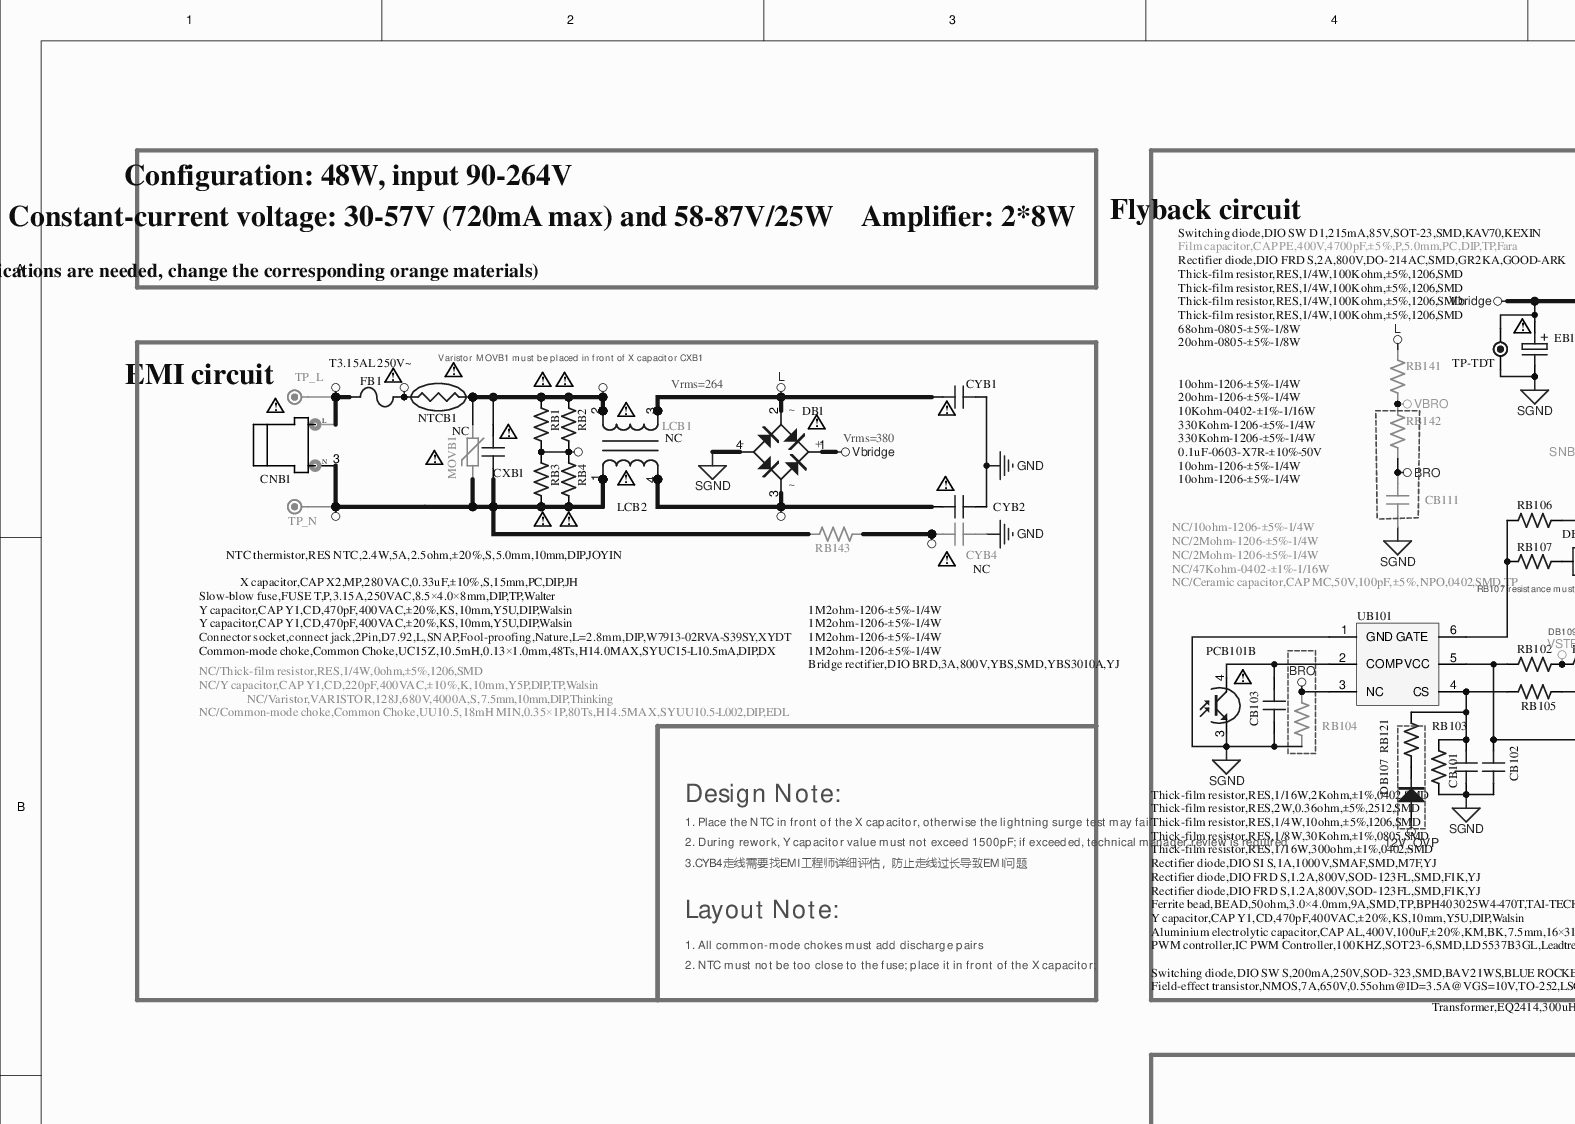
[diagram p0: MISC86372-5.SchDoc, top left]
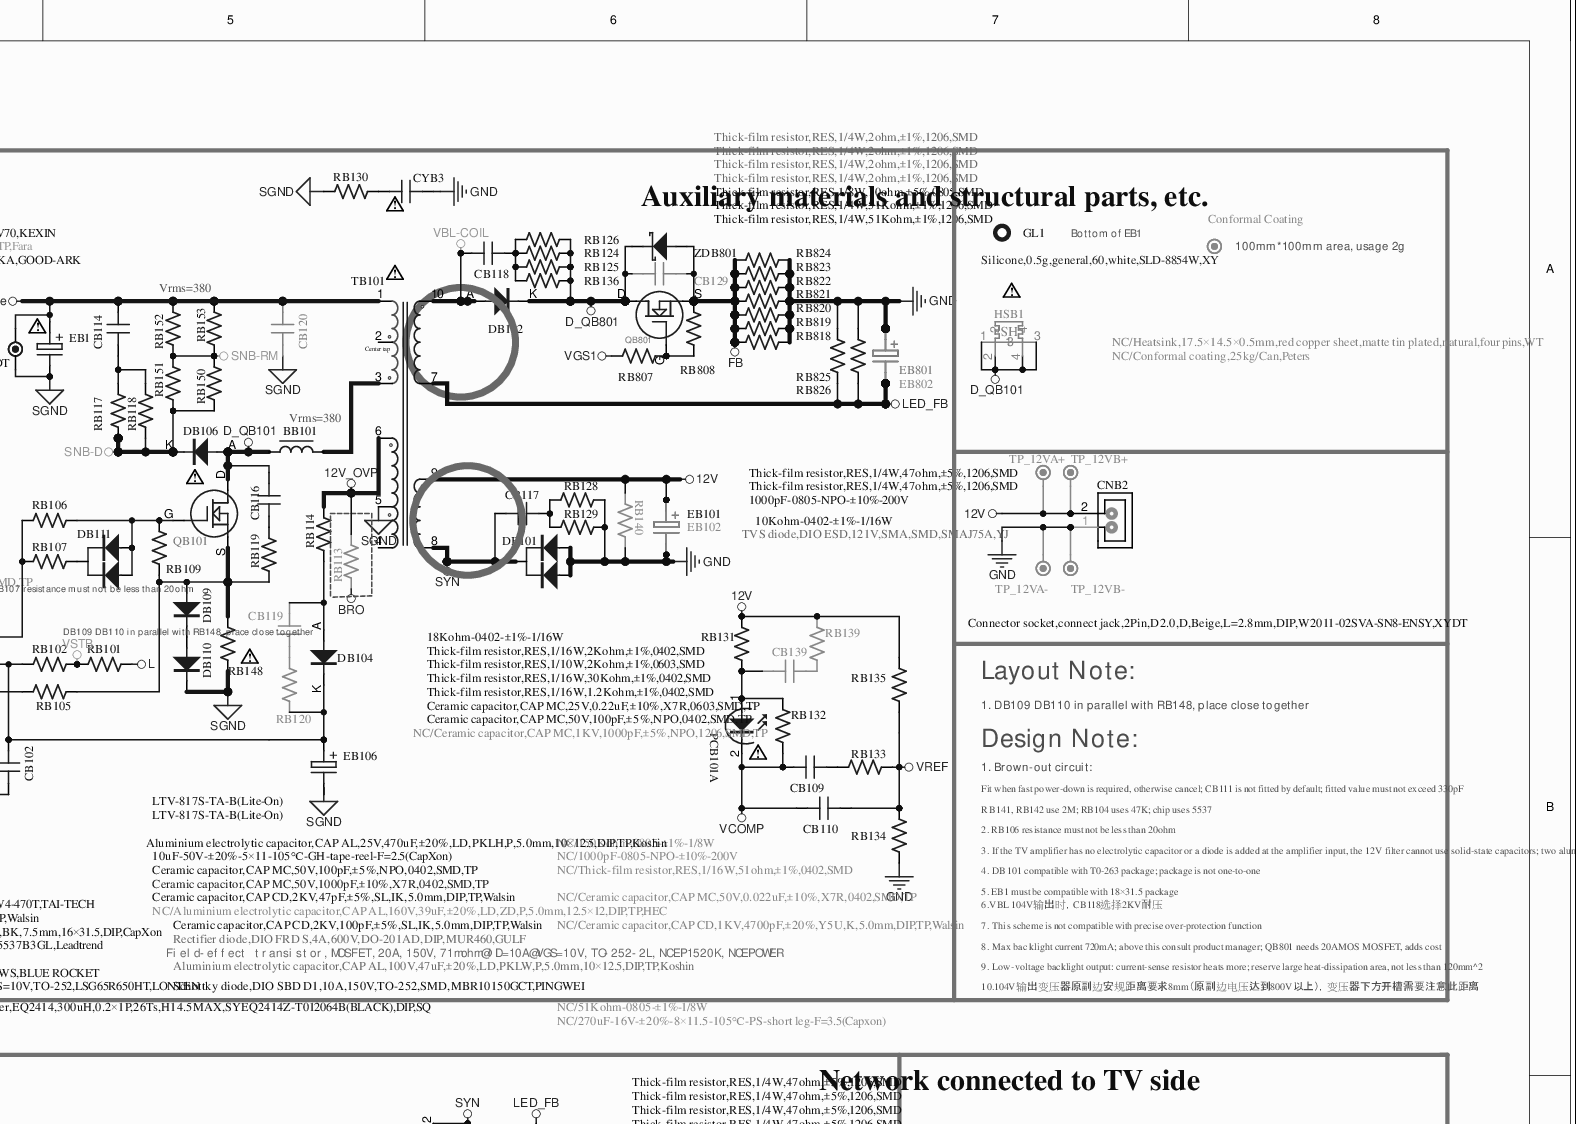
[diagram p1: MISC86372-5.SchDoc, top right]
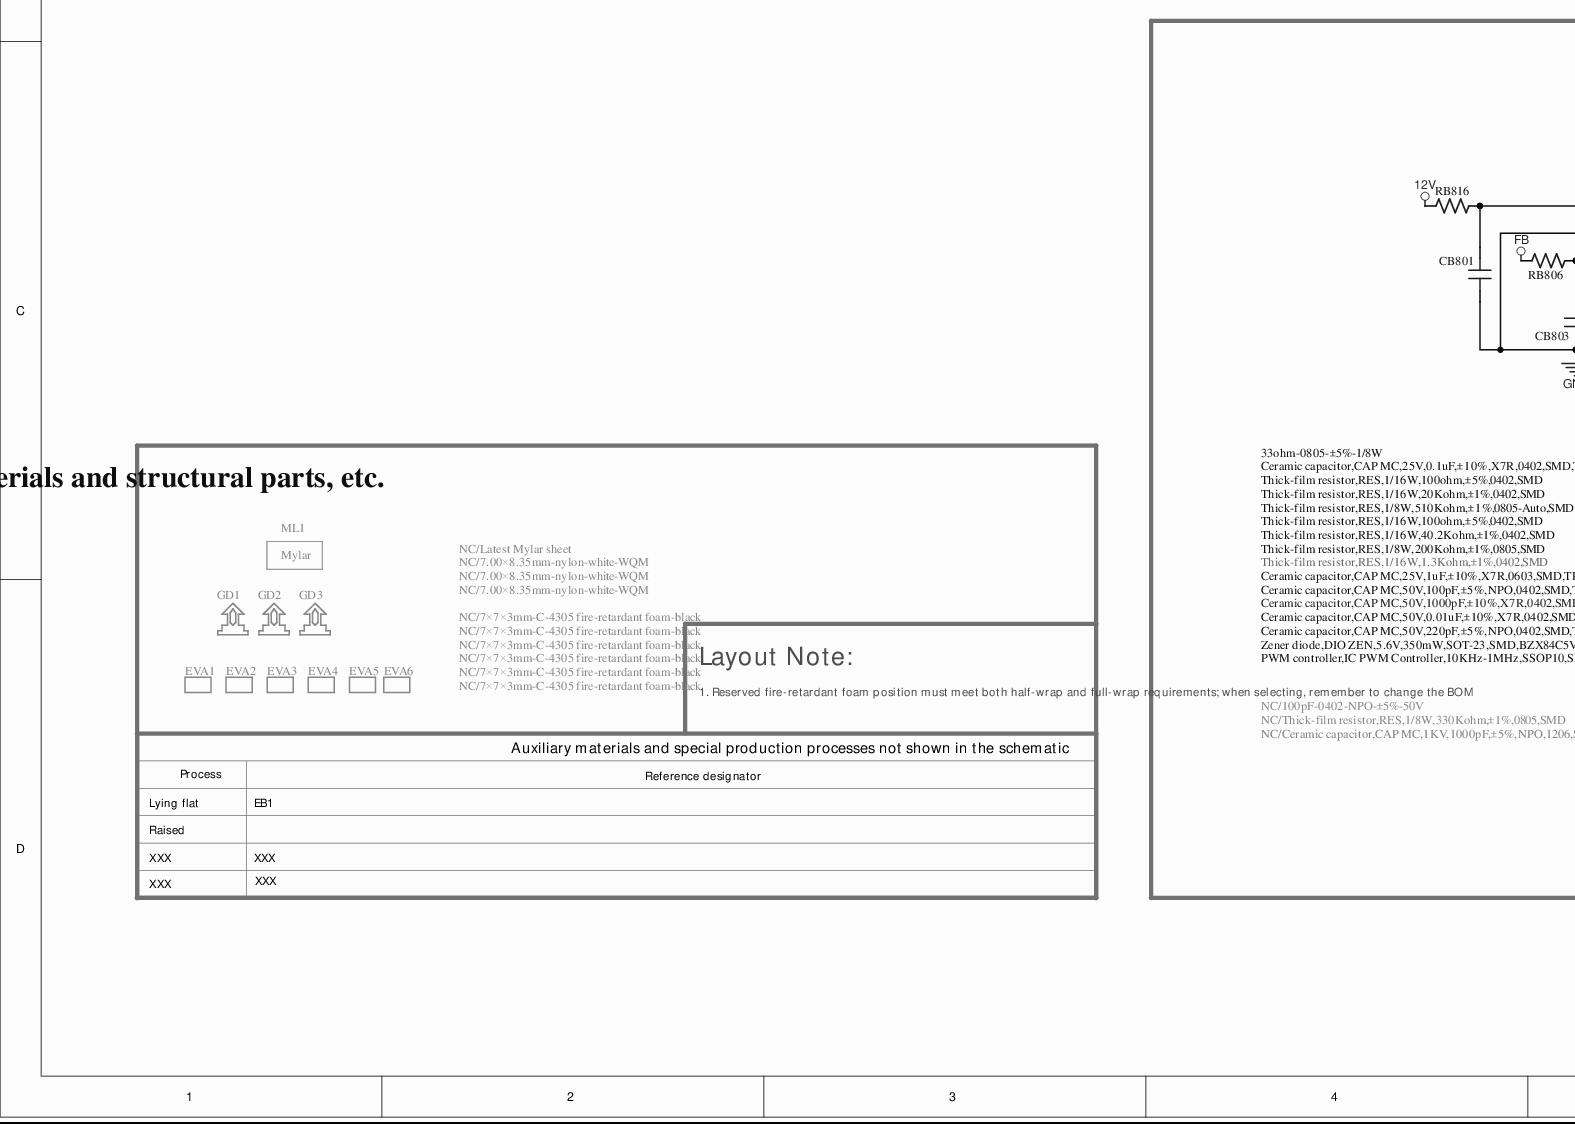
[diagram p2: MISC86372-5.SchDoc, bottom left]
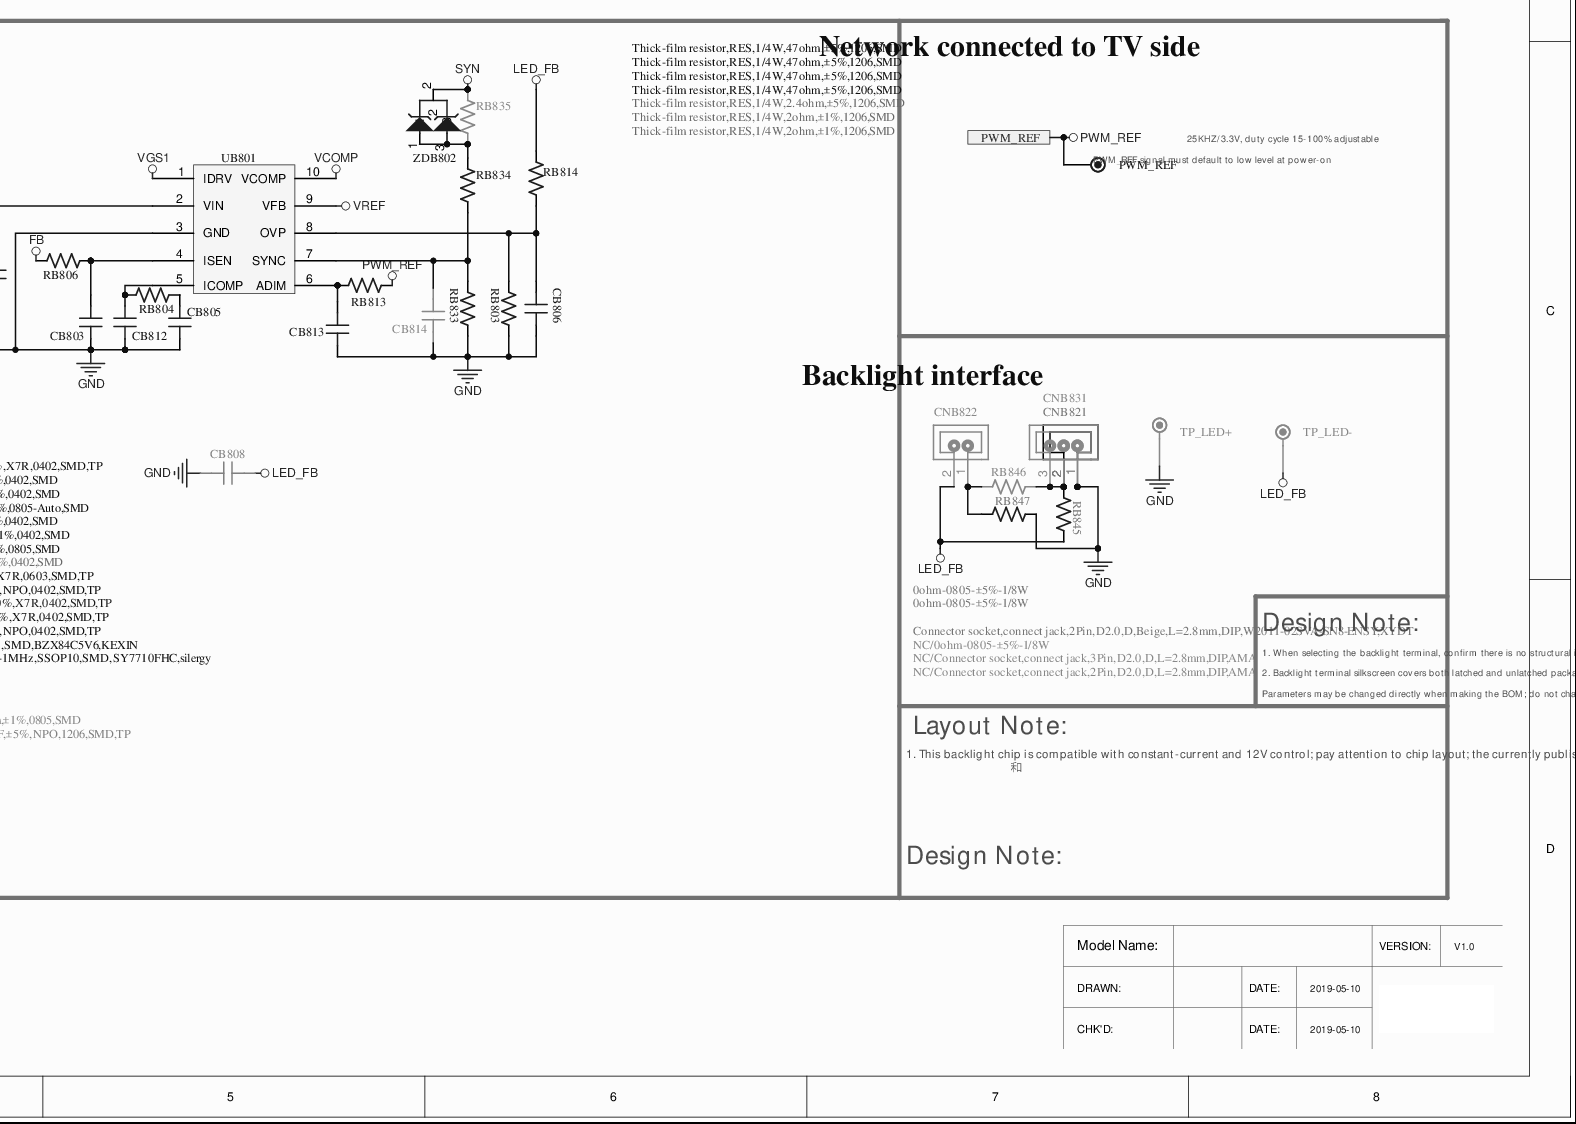
[diagram p3: MISC86372-5.SchDoc, bottom right]
# Altium project MISC86372-32.PrjPCB (part 7 of 8)

## Sheet MISC86372-5.SchDoc: MISC86372
size A2

### Parts
BB101  Ferrite bead,BEAD,50ohm,3.0×4.0mm,9A,SMD,TP,BPH403025W4-470T,TAI-TECH  [L(4*3*2.55)-S]
CB101  Ceramic capacitor,CAP MC,50V,100pF,±5%,NPO,0402,SMD,TP  [C0402]
CB102  0.1uF-0603-X7R-±10%-50V  [C0603]
CB103  Ceramic capacitor,CAP MC,50V,1000pF,±10%,X7R,0402,SMD,TP  [C0402]
CB109  Ceramic capacitor,CAP MC,25V,0.22uF,±10%,X7R,0603,SMD,TP  [C0603]
CB110  Ceramic capacitor,CAP MC,50V,100pF,±5%,NPO,0402,SMD,TP  [C0402]
CB111  NC/Ceramic capacitor,CAP MC,50V,100pF,±5%,NPO,0402,SMD,TP  [C0402]
CB114  Film capacitor,CAP PE,400V,4700pF,±5%,P,5.0mm,PC,DIP,TP,Fara  [CAP8*2.5-V-5]
CB116  Ceramic capacitor,CAP CD,2KV,47pF,±5%,SL,IK,5.0mm,DIP,TP,Walsin  [CAP7.5*5-V-5-1]
CB117  1000pF-0805-NPO-±10%-200V  [C0805]
CB118  Ceramic capacitor,CAP CD,2KV,100pF,±5%,SL,IK,5.0mm,DIP,TP,Walsin  [CAP8.5*5-V-5]
CB119  NC/1000pF-0805-NPO-±10%-200V  [C0805]
CB120  NC/Ceramic capacitor,CAP CD,1KV,4700pF,±20%,Y5U,K,5.0mm,DIP,TP,Walsin  [CAP10*4.5-V-5]
CB129  NC/Ceramic capacitor,CAP MC,1KV,1000pF,±5%,NPO,1206,SMD,TP  [C1206]
CB139  NC/Ceramic capacitor,CAP MC,50V,0.022uF,±10%,X7R,0402,SMD,TP  [C0603]
CB801  Ceramic capacitor,CAP MC,25V,1uF,±10%,X7R,0603,SMD,TP  [C0603]
CB803  Ceramic capacitor,CAP MC,25V,0.1uF,±10%,X7R,0402,SMD,TP  [C0402]
CB805  Ceramic capacitor,CAP MC,50V,0.01uF,±10%,X7R,0402,SMD,TP  [C0402]
CB806  Ceramic capacitor,CAP MC,50V,1000pF,±10%,X7R,0402,SMD,TP  [C0402]
CB808  NC/Ceramic capacitor,CAP MC,1KV,1000pF,±5%,NPO,1206,SMD,TP  [C1206]
CB812  Ceramic capacitor,CAP MC,50V,220pF,±5%,NPO,0402,SMD,TP  [C0402]
CB813  Ceramic capacitor,CAP MC,50V,100pF,±5%,NPO,0402,SMD,TP  [C0402]
CB814  NC/100pF-0402-NPO-±5%-50V  [C0402]
CNB1  Connector socket,connect jack,2Pin,D7.92,L,SNAP,Fool-proofing,Nature,L=2.8mm,DIP,W7913-02RVA-S39SY,XYDT  [CON2-H7.92]
CNB2  Connector socket,connect jack,2Pin,D2.0,D,Beige,L=2.8mm,DIP,W2011-02SVA-SN8-ENSY,XYDT  [SIP2/2.0D-1]
CNB821  Connector socket,connect jack,2Pin,D2.0,D,Beige,L=2.8mm,DIP,W2011-02SVA-SN8-ENSY,XYDT  [SIP2/2.0D-CP]
CNB822  NC/Connector socket,connect jack,2Pin,D2.0,D,L=2.8mm,DIP,AMA  [SIP2/2.0D-CP]
CNB831  NC/Connector socket,connect jack,3Pin,D2.0,D,L=2.8mm,DIP,AMA  [SIP3/2.0D-CP]
Conformal_Coating  NC/Conformal coating,25kg/Can,Peters  [Conformal Coating]
CXB1  X capacitor,CAP X2,MP,280VAC,0.33uF,±10%,S,15mm,PC,DIP,JH  [CAP18*8.5-V-15]
CYB1  Y capacitor,CAP Y1,CD,470pF,400VAC,±20%,KS,10mm,Y5U,DIP,Walsin  [CAP13*5-V-10-1]
CYB2  Y capacitor,CAP Y1,CD,470pF,400VAC,±20%,KS,10mm,Y5U,DIP,Walsin  [CAP13*5-V-10-1]
CYB3  Y capacitor,CAP Y1,CD,470pF,400VAC,±20%,KS,10mm,Y5U,DIP,Walsin  [CAP13*5-V-10-1]
CYB4  NC/Y capacitor,CAP Y1,CD,220pF,400VAC,±10%,K,10mm,Y5P,DIP,TP,Walsin  [CAP13*5-V-10-1]
DB1  Bridge rectifier,DIO BRD,3A,800V,YBS,SMD,YBS3010A,YJ  [B/YBS3010A]
DB101  Schottky diode,DIO SBD D1,10A,150V,TO-252,SMD,MBR10150GCT,PINGWEI  [D2PAK3]
DB102  Rectifier diode,DIO FRD S,4A,600V,DO-201AD,DIP,MUR460,GULF  [D3-H-20]
DB104  Rectifier diode,DIO SI S,1A,1000V,SMAF,SMD,M7F,YJ  [DIODE-S-2]
DB106  Rectifier diode,DIO FRD S,2A,800V,DO-214AC,SMD,GR2KA,GOOD-ARK  [DIODE-SMA-2]
DB107  Switching diode,DIO SW S,200mA,250V,SOD-323,SMD,BAV21WS,BLUE ROCKET  [DIODE-S-12]
DB109  Rectifier diode,DIO FRD S,1.2A,800V,SOD-123FL,SMD,F1K,YJ  [DIODE-S-14]
DB110  Rectifier diode,DIO FRD S,1.2A,800V,SOD-123FL,SMD,F1K,YJ  [DIODE-S-14]
DB111  Switching diode,DIO SW D1,215mA,85V,SOT-23,SMD,KAV70,KEXIN  [SO-23]
EB1  Aluminium electrolytic capacitor,CAP AL,400V,100uF,±20%,KM,BK,7.5mm,16×31.5,DIP,CapXon  [EC(18*31.5)-H-7.5]
EB101  Aluminium electrolytic capacitor,CAP AL,25V,470uF,±20%,LD,PKLH,P,5.0mm,10×12.5,DIP,TP,Koshin  [EC(10*12.5)-V-5]
EB102  NC/270uF-16V-±20%-8×11.5-105℃-PS-short leg-F=3.5(Capxon)  [EC(8*11)-V-3.5]
EB106  10uF-50V-±20%-5×11-105℃-GH-tape-reel-F=2.5(CapXon)  [EC(5*11)-V-2.5]
EB801  Aluminium electrolytic capacitor,CAP AL,100V,47uF,±20%,LD,PKLW,P,5.0mm,10×12.5,DIP,TP,Koshin  [EC(10*12.5)-V-5]
EB802  NC/Aluminium electrolytic capacitor,CAP AL,160V,39uF,±20%,LD,ZD,P,5.0mm,12.5×12,DIP,TP,HEC  [EC(13*13)-V-5]
EVA1  NC/7×7×3mm-C-4305 fire-retardant foam-black  [EVA(7*7*3)]
EVA2  NC/7×7×3mm-C-4305 fire-retardant foam-black  [EVA(7*7*3)]
EVA3  NC/7×7×3mm-C-4305 fire-retardant foam-black  [EVA(7*7*3)]
EVA4  NC/7×7×3mm-C-4305 fire-retardant foam-black  [EVA(7*7*3)]
EVA5  NC/7×7×3mm-C-4305 fire-retardant foam-black  [EVA(7*7*3)]
EVA6  NC/7×7×3mm-C-4305 fire-retardant foam-black  [EVA(7*7*3)]
FB1  Slow-blow fuse,FUSE T,P,3.15A,250VAC,8.5×4.0×8mm,DIP,TP,Walter  [FUSE8.5*4-V-5(T3.15AL 250V~)]
GD1  NC/7.00×8.35mm-nylon-white-WQM  [Fixed]
GD2  NC/7.00×8.35mm-nylon-white-WQM  [Fixed]
GD3  NC/7.00×8.35mm-nylon-white-WQM  [Fixed]
GL1  Silicone,0.5g,general,60,white,SLD-8854W,XY  [Silica gel-15]
HSB1  NC/Heatsink,17.5×14.5×0.5mm,red copper sheet,matte tin plated,natural,four pins,WT  [HS149-YZ]
LCB1  NC/Common-mode choke,Common Choke,UU10.5,18mH MIN,0.35×1P,80Ts,H14.5MAX,SYUU10.5-L002,DIP,EDL  [L/UU10.5/10*13-2]
LCB2  Common-mode choke,Common Choke,UC15Z,10.5mH,0.13×1.0mm,48Ts,H14.0MAX,SYUC15-L10.5mA,DIP,DX  [L/LC4/20.5*16-H-17*9(12.9)]
ML1  NC/Latest Mylar sheet  [Mylar]
MOVB1  NC/Varistor,VARISTOR,128J,680V,4000A,S,7.5mm,10mm,DIP,Thinking  [VR(13*5)-V-7.5]
NTCB1  NTC thermistor,RES NTC,2.4W,5A,2.5ohm,±20%,S,5.0mm,10mm,DIP,JOYIN  [NTC(10*5)-V5]
PCB101  LTV-817S-TA-B(Lite-On)  [OC4-S-1]  (parts A,B of 2)
PWM_REF  (no value)  [TP_BL]
QB101  Field-effect transistor,NMOS,7A,650V,0.55ohm@ID=3.5A@VGS=10V,TO-252,LSG65R650HT,LONTEN  [TO-252-GDS]
QB801  Field-effect transistor,MOSFET,20A,150V,71mohm@ID=10A@VGS=10V,TO-252-2L,NCEP1520K,NCEPOWER  [TO-252-GDS]
RB1  1M2ohm-1206-±5%-1/4W  [R1206]
RB2  1M2ohm-1206-±5%-1/4W  [R1206]
RB3  1M2ohm-1206-±5%-1/4W  [R1206]
RB4  1M2ohm-1206-±5%-1/4W  [R1206]
RB101  330Kohm-1206-±5%-1/4W  [R1206]
RB102  330Kohm-1206-±5%-1/4W  [R1206]
RB103  Thick-film resistor,RES,1/16W,2Kohm,±1%,0402,SMD  [R0402]
RB104  NC/47Kohm-0402-±1%-1/16W  [R0402]
RB105  Thick-film resistor,RES,1/16W,300ohm,±1%,0402,SMD  [R0402]
RB106  68ohm-0805-±5%-1/8W  [R0805]
RB107  20ohm-0805-±5%-1/8W  [R0805]
RB109  10Kohm-0402-±1%-1/16W  [R0402]
RB113  NC/150Kohm-0805-±1%-1/8W  [R0805]
RB114  Thick-film resistor,RES,1/4W,10ohm,±5%,1206,SMD  [R1206]
RB117  10ohm-1206-±5%-1/4W  [R1206]
RB118  10ohm-1206-±5%-1/4W  [R1206]
RB119  10ohm-1206-±5%-1/4W  [R1206]
RB120  NC/10ohm-1206-±5%-1/4W  [R1206]
RB121  Thick-film resistor,RES,1/8W,30Kohm,±1%,0805,SMD  [R0805]
RB124  Thick-film resistor,RES,1/4W,47ohm,±5%,1206,SMD  [R1206]
RB125  Thick-film resistor,RES,1/4W,47ohm,±5%,1206,SMD  [R1206]
RB126  Thick-film resistor,RES,1/4W,47ohm,±5%,1206,SMD  [R1206]
RB128  Thick-film resistor,RES,1/4W,47ohm,±5%,1206,SMD  [R1206]
RB129  Thick-film resistor,RES,1/4W,47ohm,±5%,1206,SMD  [R1206]
RB130  20ohm-1206-±5%-1/4W  [R1206]
RB131  Thick-film resistor,RES,1/10W,2Kohm,±1%,0603,SMD  [R0603]
RB132  Thick-film resistor,RES,1/16W,1.2Kohm,±1%,0402,SMD  [R0402]
RB133  Thick-film resistor,RES,1/16W,30Kohm,±1%,0402,SMD  [R0402]
RB134  Thick-film resistor,RES,1/16W,2Kohm,±1%,0402,SMD  [R0402]
RB135  18Kohm-0402-±1%-1/16W  [R0402]
RB136  Thick-film resistor,RES,1/4W,47ohm,±5%,1206,SMD  [R1206]
RB139  NC/Thick-film resistor,RES,1/16W,51ohm,±1%,0402,SMD  [R0402]
RB140  NC/51Kohm-0805-±1%-1/8W  [R0805]
RB141  NC/2Mohm-1206-±5%-1/4W  [R1206]
RB142  NC/2Mohm-1206-±5%-1/4W  [R1206]
RB143  NC/Thick-film resistor,RES,1/4W,0ohm,±5%,1206,SMD  [R1206]
RB148  Thick-film resistor,RES,2W,0.36ohm,±5%,2512,SMD  [R2512-1]
RB150  Thick-film resistor,RES,1/4W,100Kohm,±5%,1206,SMD  [R1206]
RB151  Thick-film resistor,RES,1/4W,100Kohm,±5%,1206,SMD  [R1206]
RB152  Thick-film resistor,RES,1/4W,100Kohm,±5%,1206,SMD  [R1206]
RB153  Thick-film resistor,RES,1/4W,100Kohm,±5%,1206,SMD  [R1206]
RB803  Thick-film resistor,RES,1/16W,1.3Kohm,±1%,0402,SMD  [R0402]
RB804  Thick-film resistor,RES,1/16W,20Kohm,±1%,0402,SMD  [R0402]
RB806  Thick-film resistor,RES,1/16W,100ohm,±5%,0402,SMD  [R0402]
RB807  Thick-film resistor,RES,1/8W,10ohm,±5%,0805,SMD  [R0805]
RB808  10Kohm-0402-±1%-1/16W  [R0402]
RB813  Thick-film resistor,RES,1/16W,100ohm,±5%,0402,SMD  [R0402]
RB814  Thick-film resistor,RES,1/8W,510Kohm,±1%,0805-Auto,SMD  [R0805]
RB816  33ohm-0805-±5%-1/8W  [R0805]
RB818  Thick-film resistor,RES,1/4W,2ohm,±1%,1206,SMD  [R1206]
RB819  Thick-film resistor,RES,1/4W,2ohm,±1%,1206,SMD  [R1206]
RB820  Thick-film resistor,RES,1/4W,2ohm,±1%,1206,SMD  [R1206]
RB821  Thick-film resistor,RES,1/4W,2ohm,±1%,1206,SMD  [R1206]
RB822  Thick-film resistor,RES,1/4W,2ohm,±1%,1206,SMD  [R1206]
RB823  Thick-film resistor,RES,1/4W,2ohm,±1%,1206,SMD  [R1206]
RB824  Thick-film resistor,RES,1/4W,2.4ohm,±5%,1206,SMD  [R1206]
RB825  Thick-film resistor,RES,1/4W,51Kohm,±1%,1206,SMD  [R1206]
RB826  Thick-film resistor,RES,1/4W,51Kohm,±1%,1206,SMD  [R1206]
RB833  Thick-film resistor,RES,1/16W,40.2Kohm,±1%,0402,SMD  [R0402]
RB834  Thick-film resistor,RES,1/8W,200Kohm,±1%,0805,SMD  [R0805]
RB835  NC/Thick-film resistor,RES,1/8W,330Kohm,±1%,0805,SMD  [R0805]
RB845  0ohm-0805-±5%-1/8W  [R0805]
RB846  NC/0ohm-0805-±5%-1/8W  [R0805]
RB847  0ohm-0805-±5%-1/8W  [R0805]
TB101  Transformer,EQ2414,300uH,0.2×1P,26Ts,H14.5MAX,SYEQ2414Z-T012064B(BLACK),DIP,SQ  [T/EQ2414*10]
TP-TDT  (no value)  [TP-TDT]
TP_12VA+  NC/  [TP]  (value not drawn)
TP_12VA-  NC/  [TP]  (value not drawn)
TP_12VB+  NC/  [TP]  (value not drawn)
TP_12VB-  NC/  [TP]  (value not drawn)
TP_L  NC/  [TP-80]  (value not drawn)
TP_LED+  NC/  [TP]  (value not drawn)
TP_LED-  NC/  [TP]  (value not drawn)
TP_N  NC/  [TP-80]  (value not drawn)
UB101  PWM controller,IC PWM Controller,100KHZ,SOT23-6,SMD,LD5537B3GL,Leadtrend  [SOT-26]
UB801  PWM controller,IC PWM Controller,10KHz-1MHz,SSOP10,SMD,SY7710FHC,silergy  [SOP10/1.0-1]
ZDB801  TVS diode,DIO ESD,121V,SMA,SMD,SMAJ75A,YJ  [DIODE-SMA-1]
ZDB802  Zener diode,DIO ZEN,5.6V,350mW,SOT-23,SMD,BZX84C5V6,KEXIN  [SO-23]

### Ports
PWM_REF

### Nets
12V: CNB2.2 EB101.1 EB102.1 RB131.2 RB135.1 RB139.1 RB140.1 RB816.1 TB101.9 TP_12VA+.1 TP_12VB+.1
12V_OVP: DB107.A RB113.2 RB114.2 TB101.6
BRO: CB111.2 RB104.2 RB113.1 RB142.1 UB101.3(NC)
D_QB101: BB101.1 CB116.1 DB106.A HSB1.1 HSB1.2 HSB1.3 HSB1.4 QB101.D
D_QB801: CB129.1 DB102.K QB801.D RB124.1 RB125.1 RB126.1 RB136.1 ZDB801.K
FB: CB129.2 QB801.S RB806.1 RB808.2 RB818.1 RB819.1 RB820.1 RB821.1 RB822.1 RB823.1 RB824.1 ZDB801.A
GND: CB801.2 CB803.2 CB805.1 CB806.2 CB808.1 CB812.1 CB813.1 CB814.2 CNB2.1 CNB821.1 CNB831.1 CYB1.2 CYB2.2 CYB3.2 CYB4.2 DB101.1 DB101.3 EB101.2 EB102.2 EB801.1 EB802.1 RB128.2 RB129.2 RB134.1 RB140.2 RB803.1 RB818.2 RB819.2 RB820.2 RB821.2 RB822.2 RB823.2 RB824.2 RB825.1 RB826.1 RB833.1 RB847.1 TP_12VA-.1 TP_12VB-.1 TP_LED+.1 UB801.3(GND)
L: CYB1.1 DB1.2 LCB1.3 LCB2.3 RB101.1 RB141.2
L-1: CNB1.1 FB1.1 TP_L.1
L-2: FB1.2 NTCB1.1
L-3: CXB1.1 LCB1.2 LCB2.2 MOVB1.1 NTCB1.2 RB1.1 RB2.1
L-N: RB1.2 RB2.2 RB3.1 RB4.1
LED_FB: CB808.2 CNB822.2 EB801.2 EB802.2 RB814.1 RB825.2 RB826.2 RB845.1 TB101.7 TP_LED-.1
N-1: CNB1.3 CXB1.2 LCB1.1 LCB2.1 MOVB1.2 RB3.2 RB4.2 RB143.1 TP_N.1
N-2: CYB2.1 DB1.3 LCB1.4 LCB2.4
N-3: CYB4.1 RB143.2
PWM_REF: PWM_REF.1 RB813.1 ; port PWM_REF
SGND: CB101.2 CB102.2 CB103.2 CB111.1 CB120.1 DB1.4 DB110.K EB1.2 EB106.2 PCB101.3 RB103.1 RB104.1 RB130.1 RB148.1 TB101.5 TP-TDT.2 UB101.1(GND)
SNB-D: DB106.K RB117.1 RB118.1 RB150.1 RB151.1
SNB-RM: RB150.2 RB151.2 RB152.1 RB153.1
SYN: CB117.1 DB101.2 RB835.1 TB101.8 ZDB802.2
VBL-COIL: CB118.1 DB102.A TB101.10
Vbridge: CB114.1 CB120.2 DB1.1 EB1.1 RB152.2 RB153.2 TB101.1 TP-TDT.1
VBRO: RB141.1 RB142.2
VCOMP: CB109.1 CB110.1 PCB101.2 RB132.1 UB801.10(VCOMP)
VGS1: RB807.1 UB801.1(IDRV)
VREF: CB110.2 RB133.1 RB134.2 RB135.2 UB801.9(VFB)
VSTB: RB101.2 RB102.2
NetBB101_2: BB101.2 TB101.3
NetCB101_1: CB101.1 RB103.2 RB105.1 RB121.2 UB101.4(CS)
NetCB102_1: CB102.1 DB104.K EB106.1 RB102.1 RB120.1 UB101.5(VCC)
NetCB103_1: CB103.1 PCB101.4 UB101.2(COMP)
NetCB109_2: CB109.2 RB133.2
NetCB114_2: CB114.2 RB117.2 RB118.2
NetCB116_2: CB116.2 RB119.2
NetCB117_2: CB117.2 RB128.1 RB129.1
NetCB118_2: CB118.2 RB124.2 RB125.2 RB126.2 RB136.2
NetCB119_1: CB119.1 RB120.2
NetCB119_2: CB119.2 DB104.A RB114.1
NetCB139_1: CB139.1 RB139.2
NetCB139_2: CB139.2 PCB101.1 RB131.1 RB132.2
NetCB801_1: CB801.1 RB816.2 UB801.2(VIN)
NetCB803_1: CB803.1 RB806.2 UB801.4(ISEN)
NetCB805_2: CB805.2 RB804.1
NetCB806_1: CB806.1 RB803.2 RB814.2 UB801.8(OVP)
NetCB812_2: CB812.2 RB804.2 UB801.5(ICOMP)
NetCB813_2: CB813.2 RB813.2 UB801.6(ADIM)
NetCB814_1: CB814.1 RB833.2 RB834.1 UB801.7(SYNC)
NetCNB821_2: CNB821.2 CNB831.2 CNB831.3 RB845.2 RB846.1
NetCNB822_1: CNB822.1 RB846.2 RB847.2
NetCYB3_1: CYB3.1 RB130.2
NetDB107_K: DB107.K RB121.1
NetDB109_A: DB109.A QB101.S RB105.2 RB109.1 RB119.1 RB148.2
NetDB109_K: DB109.K DB110.A
NetDB111_1: DB111.1 DB111.3 QB101.G RB106.2 RB109.2
NetDB111_2: DB111.2 RB107.2
NetQB801_G: QB801.G RB807.2 RB808.1
NetRB106_1: RB106.1 RB107.1 UB101.6(GATE)
NetRB834_2: RB834.2 RB835.2 ZDB802.1 ZDB802.3

Not connected (* = marked no-connect by the designer): TB101 2* 4*

### Layout directives
net class HOT: 12V, 12V_OVP, BRO, D_QB101, D_QB801, FB, GND, L, L-1, L-2, L-3, L-N, LED_FB, N-1, N-2, N-3, PWM_REF, SGND, SNB-D, SNB-RM, SYN, VBL-COIL, Vbridge, VBRO, VCOMP, VGS1, VREF, VSTB
net class POWER: 12V, 12V_OVP, BRO, D_QB101, D_QB801, FB, GND, L, L-1, L-2, L-3, L-N, LED_FB, N-1, N-2, N-3, PWM_REF, SGND, SNB-D, SNB-RM, SYN, VBL-COIL, Vbridge, VBRO, VCOMP, VGS1, VREF, VSTB

### Notes on the sheet
- Configuration: 48W, input 90-264V
- Constant-current voltage: 30-57V (720mA max) and 58-87V/25W
- Amplifier: 2*8W
- Flyback circuit
- (near CYB3) !
- Bottom of EB1
- Auxiliary materials and structural parts, etc.
- (near Conformal_Coating) 100mm*100mm area, usage 2g
- (If other specifications are needed, change the corresponding orange materials)
- (near EB1) !
- Vrms=380
- (near TB101) !
- !
- (near TP_L) EMI circuit
- Varistor MOVB1 must be placed in front of X capacitor CXB1
- (near NTCB1) !
- Vrms=264
- (near MOVB1) NC
- (near CXB1) !
- NC
- (near DB1) !
- (near DB1) Vrms=380
- (near CYB1) !
- (near BB101) Vrms=380
- (near RB4) !
- (near CYB2) !
- (near QB101) !
- (near CYB4) !
- (near CYB4) NC
- (near DB109) RB107 resistance must not be less than 20ohm
- DB109 DB110 in parallel with RB148, place close together
- (near RB148) !
- 1. DB109 DB110 in parallel with RB148, place close together
- Layout Note:
- Design Note:
- 1. Brown-out circuit:
- Fit when fast power-down is required, otherwise cancel; CB111 is not fitted by default; fitted value must not exceed 330pF
- RB141, RB142 use 2M; RB104 uses 47K; chip uses 5537
- 1. Place the NTC in front of the X capacitor, otherwise the lightning surge test may fail
- (near DB107) 2. During rework, Y capacitor value must not exceed 1500pF; if exceeded, technical manager review is required
- 3.CYB4走线需要找EMI工程师详细评估，防止走线过长导致EMI问题
- 3. If the TV amplifier has no electrolytic capacitor or a diode is added at the amplifier input, the 12V filter cannot use solid-state capacitors; two aluminium electrolytics are required
- 4. DB101 compatible with T0-263 package; package is not one-to-one
- 2. RB106 resistance must not be less than 20ohm
- 1. All common-mode chokes must add discharge pairs
- 6.VBL 104V输出时，CB118选择2KV耐压
- 5. EB1 must be compatible with 18×31.5 package
- 7. This scheme is not compatible with precise over-protection function
- 8. Max backlight current 720mA; above this consult product manager; QB801 needs 20AMOS MOSFET, adds cost
- 2. NTC must not be too close to the fuse; place it in front of the X capacitor;
- 9. Low-voltage backlight output: current-sense resistor heats more; reserve large heat-dissipation area, not less than 120mm^2
- 10.104V输出变压器原副边安规距离要求8mm（原副边电压达到800V以上），变压器下方开槽需要注意此距离
- Network connected to TV side
- 25KHZ/3.3V, duty cycle 15-100% adjustable
- (near PWM_REF) PWM_REF signal must default to low level at power-on
- Backlight interface
- (near ML1) Auxiliary materials and structural parts, etc.
- 1. When selecting the backlight terminal, confirm there is no structural interference with the PCB
- 1. Reserved fire-retardant foam position must meet both half-wrap and full-wrap requirements; when selecting, remember to change the BOM
- 2. Backlight terminal silkscreen covers both latched and unlatched packages
- Parameters may be changed directly when making the BOM; do not change the package
- Process
- Auxiliary materials and special production processes not shown in the schematic
- Reference designator
- 1. This backlight chip is compatible with constant-current and 12V control; pay attention to chip layout; the currently published layout scheme may be referred to
- XXXXXXXXXXXXXXXX和XXXXXXXXXXXXXX
- Lying flat
- Raised
- XXX
- EB1
- Model Name:
- DRAWN:
- XXXXXXXXXXXXXX XXXXXX
- PERSON_A
- DATE:
- 2019-05-10
- VERSION:
- V1.0
- CHK'D:
- PERSON_B
- Title
- Size:
- Date:
- A4
- Number:
- Time:
- Revision:
- Sheet
- of
- File:

### Library data of the parts
BB101 = 磁珠,BEAD,50ohm,3.0×4.0,9A,SMD,TP,SMB-302540-K5B-L1,SOLDIER-D
CB101 CB803 CB814 = 100pF-0402-NPO-±5%-50V-D
CB102 CB109 CB139 = 0.1uF-0603-X7R-±10%-50V-D: CAP
CB103 = 1000pF-0402-X7R-±10%-50V-D
CB110 CB806 = 1000pF-0402-X7R-±10%-50V-D: CAP
CB111 = 004.003.0000501-D: Ceramic capacitor,CAP MC,50V,100pF,±5%,NPO,0402,SMD,TP-D
CB114 = C242G472J20A201(编带/法拉)-DAI: CAP
CB116 = 004.003.0001895-DHAI: Ceramic capacitor,CAP CD,2KV,100pF,±5%,SL,OK,5.0mm,DIP,TP,TDK-DHAI
CB117 CB119 = 1000pF-0805-NPO-±10%-200V-D: CAP
CB118 = 004.003.0001892-DHAI: Ceramic capacitor,CAP CD,1KV,220pF,±5%,SL,OK,5.0mm,DIP,TP,TDK-DHAI
CB120 = 004.003.0001665: Ceramic capacitor,CAP CD,1KV,4700pF,±20%,Y5U,K,5.0mm,DIP,TP,Walsin-DHAI
CB129 CB808 = 22pF-1206-NPO±5%-1000V-D
CB801 = 1uf-0603-X7R-±10%-25V-D
CB805 = 0.1uF-0402-X7R-±10%-16V-D
CB812 = 0.033uF-0402-X7R-±10%-16V-D
CB813 = 4700pF-0402-X7R-±10%-50V-D
CNB1 = 连接插座,connect jack,2Pin,D7.92,L,SNAP,Fool-proofing,nature,L=2.8mm,DIP,AMA-DLMI: AC socket
CNB2 CNB821 CNB822 = XXX.XXX.0001753: Connector socket,connect jack,2Pin,D2.0,D,L=2.8mm,DIP,AMA-DHMI
CNB831 = XXX.XXX.0001754: Connector socket,connect jack,3Pin,D2.0,D,L=2.8mm,DIP,AMA-DHMI
Conformal_Coating = 三防漆,25kg/Can,Peters
CXB1 = X电容,CAP X2,MP,275VAC,0.47uF,±10%,S,15mm-Mini,PC,DIP,BM-DHMI: CAP
CYB1-CYB4 = Y电容,CAP Y1,CD,470pF,400VAC,±20%,KS,10mm,Y5U,DIP,Walsin-DHMI: Y1 capacitor
DB1 = 004.005.0000860-D: Bridge rectifier,DIO BRD,3A,800V,YBS,SMD,YBS3010A,YJ-D
DB101 = MBRB10150CT(GOOD-ARK)-D: Diode
DB102 = 004.005.0000308: Rectifier diode,DIO UFRD S,4A,800V,DO-201AD,DIP,MUR480ERLG,ON-DLMI
DB104 = M7(WEJ)-D: Diode
DB106 = 004.005.0000504-D: Rectifier diode,DIO FRD S,2A,800V,DO-214AC,SMD,GR2KA,GOOD-ARK-D
DB107 = BAV21WS-D: Diode
DB109 DB110 = 整流二极管,DIO FRD S,1.2A,800V,eSGA,SMD,R12K,GOOD-ARK-D
DB111 = LBAV70LT1G(LRC)-D: Diode
EB1 = 铝电解电容,CAP AL,450V,68uF,±20%,KM,BK,7.5mm,18×31.5,DIP,CapXon-DLMI: CAP
EB101 = 470uF-25V-±20%-10×12.5-105℃-GF-编带-F=5.0(CapXon)-DHAI: Electrolytic
EB102 = 270uF-16V-±20%-8×11.5-105℃-PS-短脚-F=3.5(Capxon): Solid-state
EB106 = 10uF-50V-±20%-5×11-105℃-GH-编带-F=2.5(CapXon)-DHAI: Electrolytic
EB801 = 004.003.0000876: Aluminium electrolytic capacitor,CAP AL,100V,47uF,±20%,LD,SK,P,5.0mm,10×12.5,DIP,TP,Samxon-DHAI
EB802 = 004.003.0000945: Aluminium electrolytic capacitor,CAP AL,160V,39uF,±20%,LD,DV,P,5.0mm,12.5×12,DIP,TP,Elite-DHAI
EVA1-EVA6 = 7×7×3mm-C-4305防火泡棉-黑色-DLMI: EVA
FB1 = 004.026.0000010-DHMI: Slow-blow fuse,FUSE T,P,3.15A,250VAC,8.5×4.0×8mm,DIP,TP,Walter-DHMI
GD1-GD3 = 7.00×8.35mm-尼龙-白色-WQM-DHMI: Mylar standoff
GL1 = 005.002.0000011: Silicone,0.2g,general,60,white,SLD-8854W,XY-DHMI
HSB1 = 004.040.0006600-DHMI: Heatsink,17.5×14.5×0.5mm,red copper sheet,matte tin plated,natural,four pins,WT-DHMI
LCB1 = SYUU10.5-L002-JM-DHMI: Common-mode choke
LCB2 = 共模电感,Common Choke,UC15,10.5mH,0.13×1.0mm,48Ts,H14.0MAX,SYUC15-L10.5mA,DIP,UENO-DLMI: Common-mode choke
ML1 = MALAY
MOVB1 = TVR10561KSW(为勤)-DHMI: Varistor
NTCB1 = SCK102R55AMBY502(短脚/为勤)-DHMI: Thermistor
PCB101 = LTV-817S-TA-B(光宝)-DMI: Optocoupler
PWM_REF TP-TDT TP_12VA+ TP_12VA- TP_12VB+ TP_12VB- TP_L TP_LED+ TP_LED- TP_N = TEST
QB101 = 场效应管,NMOS,5.2,650V,1.02ohm@ID=2.6A@VGS=10V,DPAK,TK5P65W,TOSHIBA-D: N Channel Single MOSFET
QB801 = ME15N10(松木)-D: N Channel Single MOSFET
RB1-RB4 = 1M2ohm-1206-±5%-1/4W-D: RES
RB101 RB102 = 330Kohm-1206-±5%-1/4W-D: RES
RB103 RB109 RB808 = 10Kohm-0402-±1%-1/16W-D
RB104 = 47Kohm-0402-±1%-1/16W-D
RB105 = 510ohm-0402-±1%-1/16W-D
RB106 RB113 RB121 = 68ohm-0805-±5%-1/8W-D
RB107 RB807 = 20ohm-0805-±5%-1/8W-D: RES
RB114 = 4R7ohm-1206-±1%-1/4W-D: RES
RB117-RB120 = 10ohm-1206-±5%-1/4W-D: RES
RB124-RB126 RB136 = 68ohm-1206-±5%-1/4W-D
RB128 RB129 = 47ohm-1206-±5%-1/4W-D: RES
RB130 RB143 = 20ohm-1206-±5%-1/4W-D
RB131 = 2Kohm-0603-±5%-1/10W-D
RB132 RB133 RB139 = 3Kohm-0402-±1%-1/16W-D
RB134 = 4K7ohm-0402-±1%-1/16W-D: RES
RB135 = 18Kohm-0402-±1%-1/16W-D: RES
RB140 = 51Kohm-0805-±1%-1/8W-D: RES
RB141 RB142 = 2Mohm-1206-±5%-1/4W-D: RES
RB148 = 厚膜电阻,RES,1W,0.24ohm,±1%,2512,SMD
RB150-RB153 RB825 RB826 = 100Kohm-1206-±5%-1/4W-D: RES
RB803 RB813 RB833 = 100ohm-0402-±5%-1/16W-D: RES
RB804 = 10Kohm-0402-±5%-1/16W-D
RB806 = 1Kohm-0402-±1%-1/16W-D
RB814 RB816 RB834 RB835 = 33ohm-0805-±5%-1/8W-D
RB818-RB824 = 0R47ohm-1206-±1%-1/4W-D
RB845-RB847 = 0ohm-0805-±5%-1/8W-D
TB101 = 004.004.0002645-DLMI: Transformer,EQ2414,300uH,0.2×1P,26Ts,H14.5MAX,SYEQ2414Z-T012064B(BLACK),DIP,SQ-DLMI
UB101 = 004.010.0000426: PWM controller,IC PWM Controller,65KHZ,SOT23-6,SMD,OB2273C,ON-Bright-D
UB801 = SY7710FHC: SSOP10
ZDB801 = TVS管,DIO ESD,400pF,24.4V,SMB,SMD,SMBJ15AHR4G,TSC-D: TVS
ZDB802 = BZX84C24(蓝箭)-D: Diode